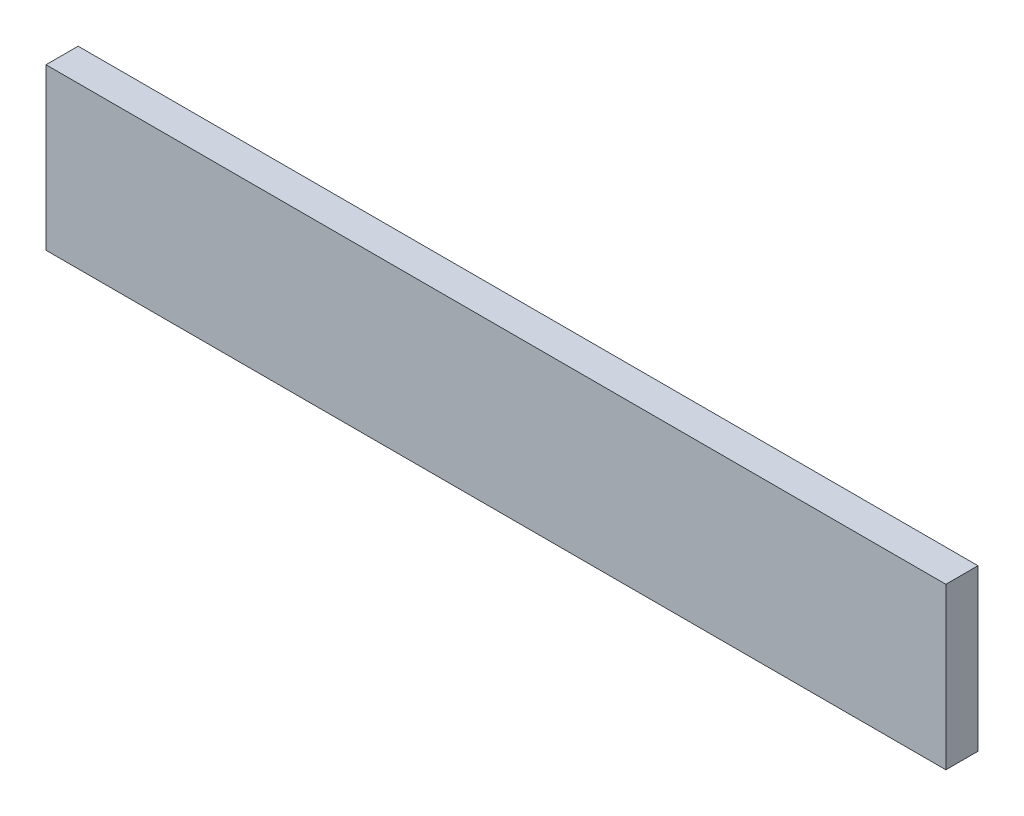
from build123d import *

# Parameters (mm, degrees)
SKETCH_1_W      = 140
SKETCH_1_H      = 25
EXTRUDE_1_DEPTH = 5


with BuildPart() as part:
    # 草图1 → 凸台-拉伸1 (new body)
    with BuildSketch(Plane.XY):
        Rectangle(SKETCH_1_W, SKETCH_1_H)
    extrude(amount=EXTRUDE_1_DEPTH)


solid = part.part
